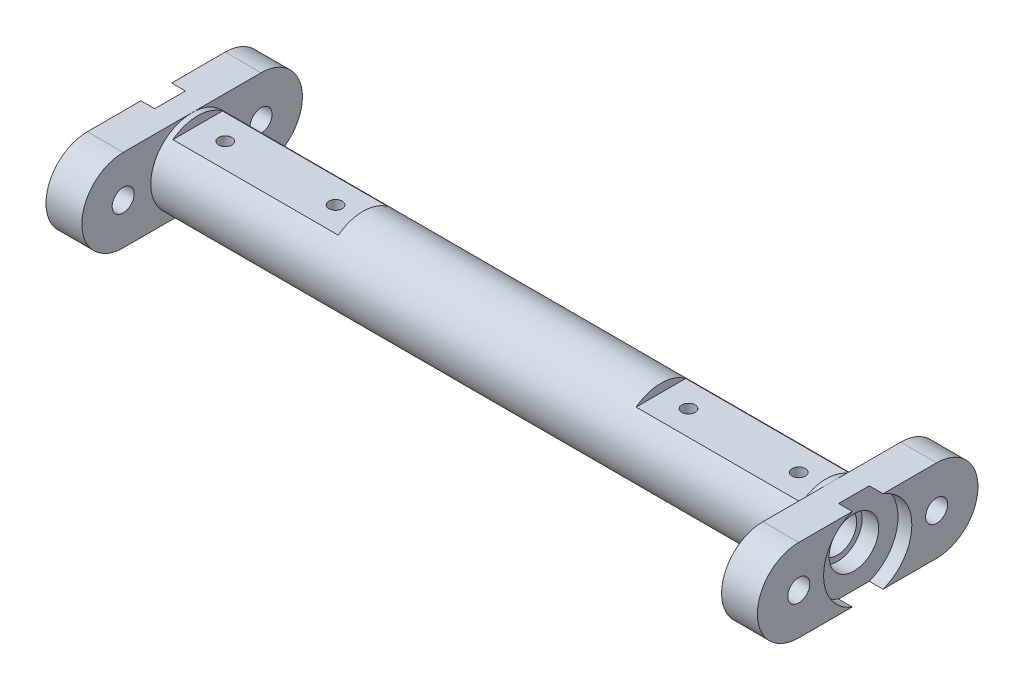
from build123d import *

# Parameters (mm, degrees)
CUT_EXTRUDE_1_DEPTH      = 630.007154172
CUT_EXTRUDE_1_DEPTH_BACK = 630.007154172
SKETCH_2_W               = 300
SKETCH_2_H               = 15
CUT_EXTRUDE_2_REACH      = 640.944
CUT_EXTRUDE_2_END_RADIUS = 35
SKETCH_3_R               = 12
SKETCH_4_R               = 20
SKETCH_4_R_2             = 45
BOSS_EXTRUDE_1_DEPTH     = 40
BOSS_EXTRUDE_START       = 25
SKETCH_5_R               = 20
BOSS_EXTRUDE_2_DEPTH     = 25


with BuildPart() as part:
    # Sketch 1 → Revolve 1 (revolve)
    with BuildSketch(Plane.XY, mode=Mode.PRIVATE) as revolve_1_sk:
        Polygon((590, 35), (-590, 35), (-590, 45), (-620, 45), (-620, 75), (620, 75), (620, 45), (590, 45), align=None)
    revolve(revolve_1_sk.sketch.rotate(Axis((-862.857142857, 0, 0), (1, 0, 0)), 90), axis=Axis((-862.857142857, 0, 0), (1, 0, 0)))

    # Sketch 2 → Cut-Extrude 1 (cut, two sides: drawn at the far end of the back side and taken through both)
    with BuildSketch(Plane.XY.offset(-CUT_EXTRUDE_1_DEPTH_BACK)):
        with Locations((-420, 67.5)):
            Rectangle(SKETCH_2_W, SKETCH_2_H)
        with Locations((420, 67.5)):
            Rectangle(SKETCH_2_W, SKETCH_2_H)
    extrude(amount=CUT_EXTRUDE_1_DEPTH + CUT_EXTRUDE_1_DEPTH_BACK, mode=Mode.SUBTRACT)

    # Cut-Extrude 2: up to this cylinder (the profile starts outside it)
    cut_extrude_2_end = Plane(origin=(0, 0, 0), z_dir=(-1, 0, 0)) * Cylinder(CUT_EXTRUDE_2_END_RADIUS, 2392.888, mode=Mode.PRIVATE)
    # Sketch 3 → Cut-Extrude 2 (cut, up to the surface)
    with BuildSketch(Plane(origin=(0, 60, 0), x_dir=(1, 0, 0), z_dir=(0, 1, 0)), mode=Mode.PRIVATE) as cut_extrude_2_sk1:
        with Locations(Location((-320, 0, 0), (0, 0, 180))):
            Circle(SKETCH_3_R)
    cut_extrude_2_tool1 = extrude(cut_extrude_2_sk1.sketch, amount=-CUT_EXTRUDE_2_REACH, mode=Mode.PRIVATE) - cut_extrude_2_end
    add(cut_extrude_2_tool1.solids().sort_by_distance((-320, 60, 0))[0], mode=Mode.SUBTRACT)
    # Sketch 3 → Cut-Extrude 2 (cut, up to the surface)
    with BuildSketch(Plane(origin=(0, 60, 0), x_dir=(1, 0, 0), z_dir=(0, 1, 0)), mode=Mode.PRIVATE) as cut_extrude_2_sk2:
        with Locations(Location((-520, 0, 0), (0, 0, 180))):
            Circle(SKETCH_3_R)
    cut_extrude_2_tool2 = extrude(cut_extrude_2_sk2.sketch, amount=-CUT_EXTRUDE_2_REACH, mode=Mode.PRIVATE) - cut_extrude_2_end
    add(cut_extrude_2_tool2.solids().sort_by_distance((-520, 60, 0))[0], mode=Mode.SUBTRACT)
    # Sketch 3 → Cut-Extrude 2 (cut, up to the surface)
    with BuildSketch(Plane(origin=(0, 60, 0), x_dir=(1, 0, 0), z_dir=(0, 1, 0)), mode=Mode.PRIVATE) as cut_extrude_2_sk3:
        with Locations(Location((520, 0, 0), (0, 0, 180))):
            Circle(SKETCH_3_R)
    cut_extrude_2_tool3 = extrude(cut_extrude_2_sk3.sketch, amount=-CUT_EXTRUDE_2_REACH, mode=Mode.PRIVATE) - cut_extrude_2_end
    add(cut_extrude_2_tool3.solids().sort_by_distance((520, 60, 0))[0], mode=Mode.SUBTRACT)
    # Sketch 3 → Cut-Extrude 2 (cut, up to the surface)
    with BuildSketch(Plane(origin=(0, 60, 0), x_dir=(1, 0, 0), z_dir=(0, 1, 0)), mode=Mode.PRIVATE) as cut_extrude_2_sk4:
        with Locations(Location((320, 0, 0), (0, 0, 180))):
            Circle(SKETCH_3_R)
    cut_extrude_2_tool4 = extrude(cut_extrude_2_sk4.sketch, amount=-CUT_EXTRUDE_2_REACH, mode=Mode.PRIVATE) - cut_extrude_2_end
    add(cut_extrude_2_tool4.solids().sort_by_distance((320, 60, 0))[0], mode=Mode.SUBTRACT)

    # Sketch 4 → Boss-Extrude 1 (add)
    with BuildSketch(Plane.ZY.offset(620)):
        with BuildLine():
            Line((-125, 75), (125, 75))
            ThreePointArc((125, 75), (200, 0), (125, -75))
            Line((125, -75), (-125, -75))
            ThreePointArc((-125, -75), (-200, 0), (-125, 75))
        make_face()
        with Locations((-125, 0)):
            Circle(SKETCH_4_R, mode=Mode.SUBTRACT)
        with Locations(Location((125, 0, 0), (0, 0, 180))):
            Circle(SKETCH_4_R, mode=Mode.SUBTRACT)
        Circle(SKETCH_4_R_2, mode=Mode.SUBTRACT)
    boss_extrude_1 = extrude(amount=-BOSS_EXTRUDE_1_DEPTH)

    # Sketch 5 → Boss-Extrude 2 (add)
    # profile 1 of 2: a face of its own
    with BuildSketch(Plane.ZY.offset(620).offset(BOSS_EXTRUDE_START)):
        with BuildLine():
            Line((-27.838821814, 75), (-125, 75))
            ThreePointArc((-125, 75), (-200, 0), (-125, -75))
            Line((-125, -75), (-27.838821814, -75))
            ThreePointArc((-27.838821814, -75), (-80, 0), (-27.838821814, 75))
        make_face()
        with Locations((-125, 0)):
            Circle(SKETCH_5_R, mode=Mode.SUBTRACT)
    # profile 2 of 2: a face of its own
    with BuildSketch(Plane.ZY.offset(620).offset(BOSS_EXTRUDE_START)):
        with BuildLine():
            Line((125, -75), (27.838821814, -75))
            ThreePointArc((27.838821814, -75), (80, 0), (27.838821814, 75))
            Line((27.838821814, 75), (125, 75))
            ThreePointArc((125, 75), (200, 0), (125, -75))
        make_face()
        with Locations(Location((125, 0, 0), (0, 0, 180))):
            Circle(SKETCH_5_R, mode=Mode.SUBTRACT)
    boss_extrude_2 = extrude(amount=-BOSS_EXTRUDE_2_DEPTH)

    # Mirror 1: Boss-Extrude 1, Boss-Extrude 2 across plane
    add(boss_extrude_1.mirror(Plane(origin=(0, 0, 0), x_dir=(0, 0, 1), z_dir=(1, 0, 0))))
    add(boss_extrude_2.mirror(Plane(origin=(0, 0, 0), x_dir=(0, 0, 1), z_dir=(1, 0, 0))))


solid = part.part
